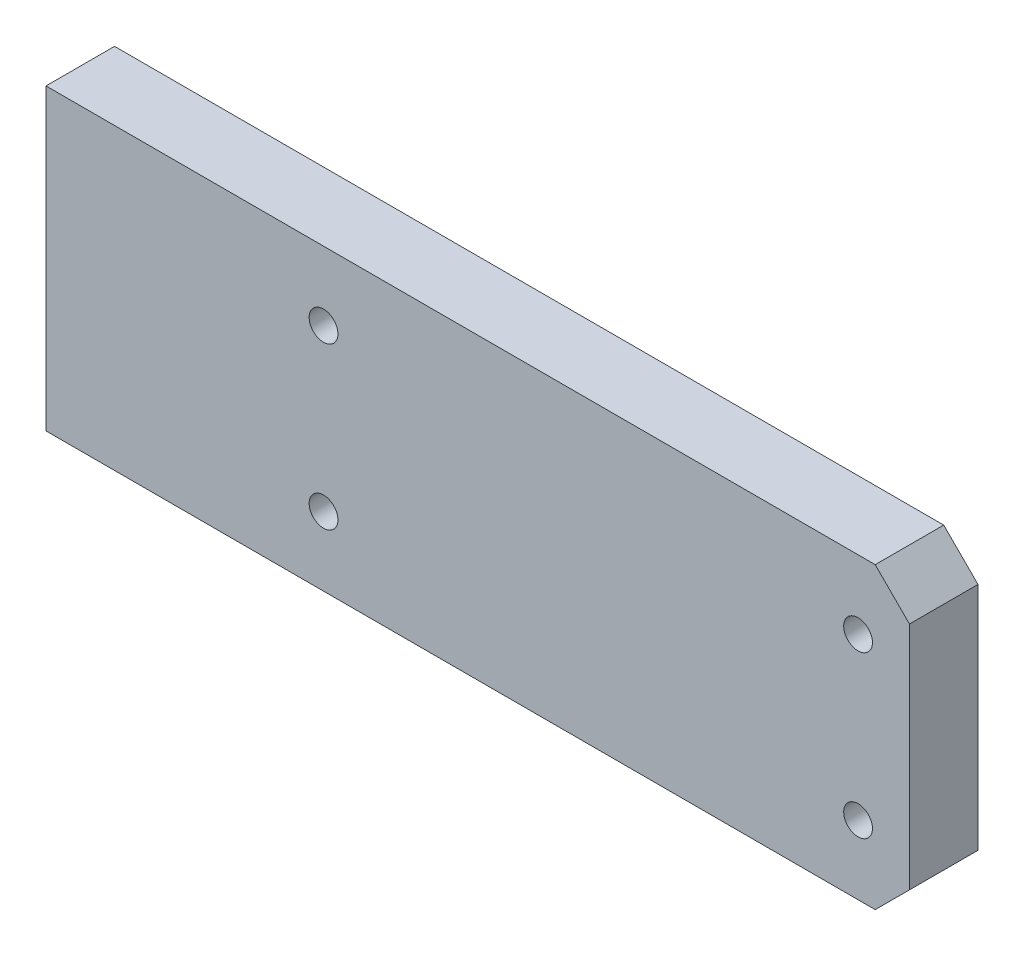
from build123d import *

# Parameters (mm, degrees)
SKETCH_1_W             = 126
SKETCH_1_H             = 10
EXTRUDE_1_DEPTH        = 43.6
CHAMFER_1_SIZE         = 5
HOLE_WIZARD_M4_1_D     = 3.3
HOLE_WIZARD_M4_1_DEPTH = 10.1
HOLE_WIZARD_M4_1_TIP   = 0.991420021
HOLE_WIZARD_M5_1_D     = 4.2


with BuildPart() as part:
    # 草图1 → 凸台-拉伸1 (new body)
    with BuildSketch(Plane(origin=(0, 0, 0), x_dir=(1, 0, 0), z_dir=(0, 1, 0))):
        with Locations((63, 5)):
            Rectangle(SKETCH_1_W, SKETCH_1_H)
    extrude(amount=EXTRUDE_1_DEPTH)

    # 倒角1
    chamfer_1_edges = [part.edges().sort_by_distance(p)[0] for p in [
        (126, 43.6, -5),
        (126, 0, -5),
    ]]
    chamfer(chamfer_1_edges, length=CHAMFER_1_SIZE)

    # M4 螺纹孔1
    with Locations(Plane.ZY):
        with Locations((-5, 36.8), (-5, 21.783451384), (-5, 6.8)):
            Hole(HOLE_WIZARD_M4_1_D / 2, depth=HOLE_WIZARD_M4_1_DEPTH)
            with Locations((0, 0, -(HOLE_WIZARD_M4_1_DEPTH + HOLE_WIZARD_M4_1_TIP / 2))):  # 118° drill point
                Cone(0, HOLE_WIZARD_M4_1_D / 2, HOLE_WIZARD_M4_1_TIP, mode=Mode.SUBTRACT)

    # M5 螺纹孔1 (through all)
    with Locations(Plane(origin=(0, 0, -10), x_dir=(-1, 0, 0), z_dir=(0, 0, -1))):
        with Locations((-40.5, 33.55), (-40.5, 10.05), (-118.5, 33.55), (-118.5, 10.05)):
            Hole(HOLE_WIZARD_M5_1_D / 2)


solid = part.part
